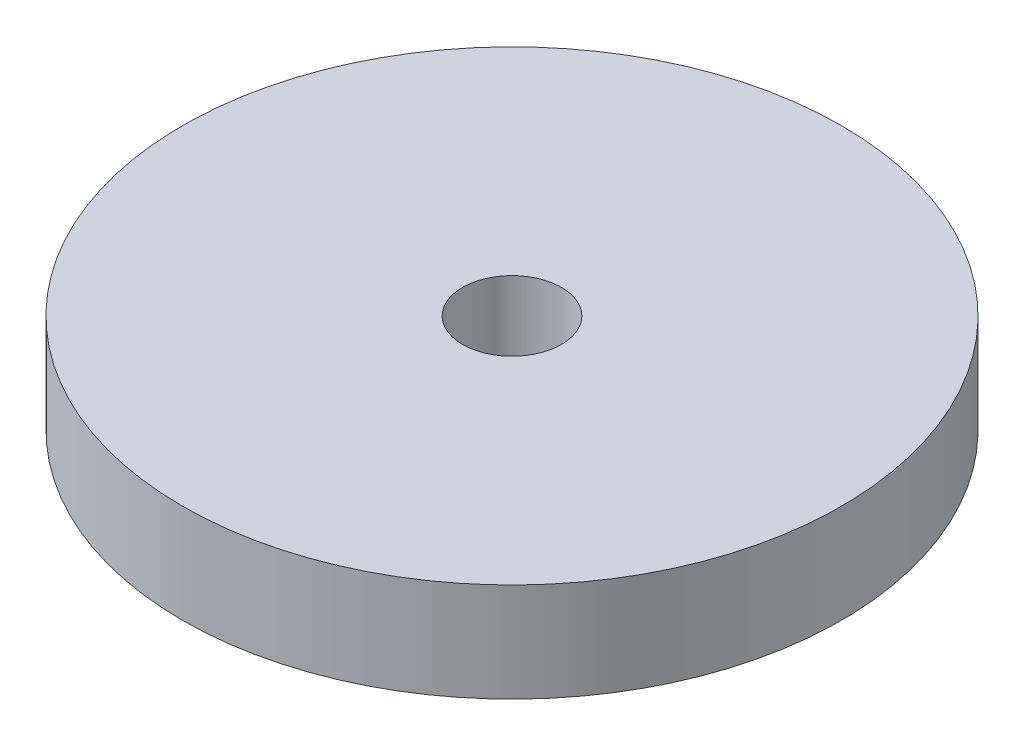
from build123d import *

# Parameters (mm, degrees)
SKETCH_1_W = 85
SKETCH_1_H = 30


with BuildPart() as part:
    # 草图1 → 旋转2 (revolve)
    with BuildSketch(Plane(origin=(0, 0, 0), x_dir=(0, 0, -1), z_dir=(1, 0, 0)), mode=Mode.PRIVATE) as revolve_2_sk:
        with Locations((57.5, 15)):
            Rectangle(SKETCH_1_W, SKETCH_1_H)
    revolve(revolve_2_sk.sketch.rotate(Axis((0, 36.72, 0), (0, -1, 0)), 180), axis=Axis((0, 36.72, 0), (0, -1, 0)))


solid = part.part
